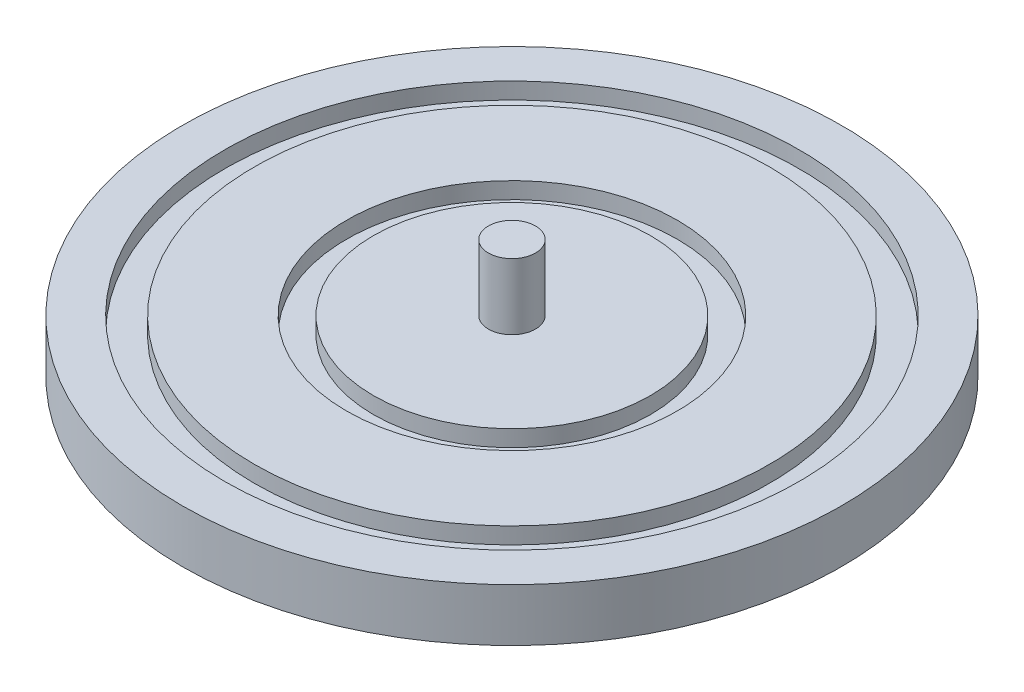
SolidWorks part; units mm, degrees
ref_plane "前视基准面" through (0, 0, 0) normal (0, 0, 1) x (1, 0, 0)
ref_plane "上视基准面" through (0, 0, 0) normal (0, 1, 0) x (1, 0, 0)
ref_plane "右视基准面" through (0, 0, 0) normal (1, 0, 0) x (0, 0, -1)
sketch "草图1" plane through (0, 0, 0) normal (0, 1, 0) x (1, 0, 0)
  circle A0 centre (0, 0) radius 20
  dimension "D1" = 40
extrude "凸台-拉伸1" add sketch "草图1" along normal blind 3.2
sketch "草图2" plane through (0, 0, 0) normal (0, -1, 0) x (1, 0, 0)
  circle A0 centre (0, 0) radius 5
  dimension "D1" = 10
extrude "凸台-拉伸2" add sketch "草图2" along normal blind 6
sketch "草图3" plane through (0, 0, 0) normal (0, -1, 0) x (1, 0, 0)
  circle A0 centre (0, 0) radius 9.5454
  circle A1 centre (0, 0) radius 11.6695
extrude "切除-拉伸1" cut sketch "草图3" against normal blind 1
sketch "草图4" plane through (0, 3.2, 0) normal (0, 1, 0) x (1, 0, 0)
  circle A0 centre (0, 0) radius 1.425
  dimension "D1" = 2.85
extrude "凸台-拉伸3" add sketch "草图4" along normal blind 4
sketch "草图5" plane through (0, 3.2, 0) normal (0, 1, 0) x (1, 0, 0)
  circle A0 centre (0, 0) radius 17.4353
  circle A1 centre (0, 0) radius 15.6342
extrude "切除-拉伸2" cut sketch "草图5" against normal blind 1
sketch "草图6" plane through (0, 3.2, 0) normal (0, 1, 0) x (1, 0, 0)
  circle A0 centre (0, 0) radius 10.0341
  circle A1 centre (0, 0) radius 8.4089
extrude "切除-拉伸3" cut sketch "草图6" against normal blind 1
